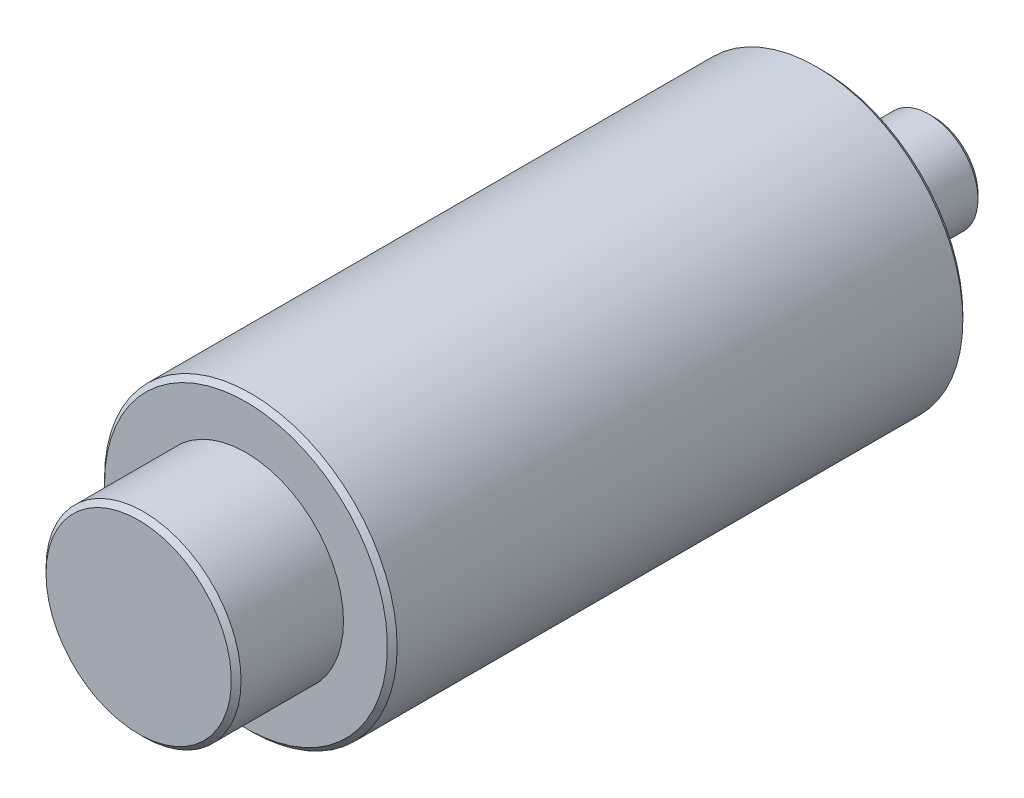
SolidWorks part; units mm, degrees
material "Q235B"
ref_plane "Front Plane" through (0, 0, 0) normal (0, 0, 1) x (1, 0, 0)
ref_plane "Top Plane" through (0, 0, 0) normal (0, 1, 0) x (1, 0, 0)
ref_plane "Right Plane" through (0, 0, 0) normal (1, 0, 0) x (0, 0, -1)
sketch "Sketch1" plane through (0, 0, 0) normal (1, 0, 0) x (0, 0, -1)
  line L0 (0, 0) -> (81.5, 0) construction
  line L1 (81.5, 0) -> (81.5, 5.05)
  line L2 (81.5, 5.05) -> (73.5, 5.05)
  line L3 (73.5, 5.05) -> (73.5, 7.5)
  line L4 (73.5, 7.5) -> (70, 7.5)
  line L5 (70, 7.5) -> (70, 15)
  line L6 (70, 15) -> (11, 15)
  line L7 (11, 15) -> (11, 10)
  line L8 (11, 10) -> (0, 10)
  line L9 (0, 10) -> (0, 0)
  line L10 (0, 0) -> (81.5, 0)
  dimension "D1" = 20
  dimension "D2" = 11
  dimension "D3" = 59
  dimension "D4" = 30
  dimension "D5" = 15
  dimension "D6" = 3.5
  dimension "D7" = 8
  dimension "D8" = 10.1
revolve "Revolve1" add sketch "Sketch1" angle 360 about L0
chamfer "Chamfer1" distance 0.5 angle 45 5 edges at (5.05, 0, -81.5) (7.5, 0, -73.5) (15, 0, -70) (15, 0, -11) (10, 0, 0)
